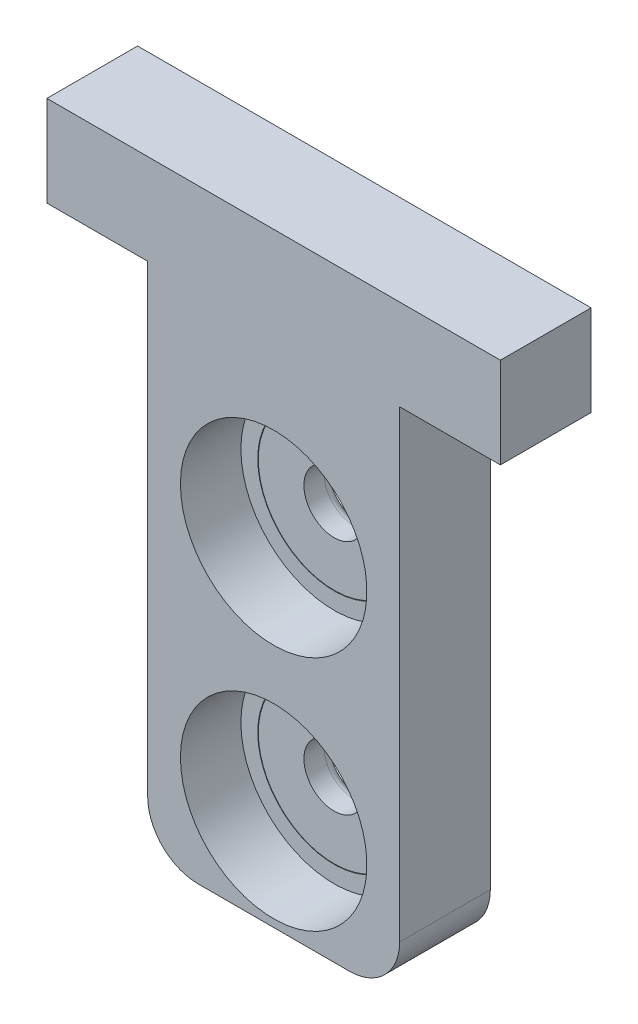
SolidWorks part; units mm, degrees
ref_plane "前视基准面" through (0, 0, 0) normal (0, 0, 1) x (1, 0, 0)
ref_plane "上视基准面" through (0, 0, 0) normal (0, 1, 0) x (1, 0, 0)
ref_plane "右视基准面" through (0, 0, 0) normal (1, 0, 0) x (0, 0, -1)
sketch "草图1" plane through (0, 0, 0) normal (0, 0, 1) x (1, 0, 0)
  line L1 (25, 60) -> (-25, 60)
  line L2 (25, 60) -> (25, -60)
  line L3 (25, -60) -> (-25, -60)
  line L4 (-25, 60) -> (-25, -60)
  line L5 (25, 60) -> (-25, -60) construction
  line L6 (25, -60) -> (-25, 60) construction
  point P0 (0, 0)
  dimension "D1" = 120
  dimension "D2" = 50
extrude "凸台-拉伸1" add sketch "草图1" along normal blind 18
sketch "草图2" plane through (0, 60, 0) normal (0, 1, 0) x (1, 0, 0)
  line L0 (25, 0) -> (-25, 0) construction
  line L1 (45, -18) -> (-45, -18)
  line L2 (45, -18) -> (45, 0)
  line L3 (45, 0) -> (-45, 0)
  line L4 (-45, -18) -> (-45, 0)
  line L5 (45, -18) -> (-45, 0) construction
  line L6 (45, 0) -> (-45, -18) construction
  line L7 (25, -18) -> (-25, -18) construction
  line L8 (0, -9) -> (0, 0) construction
  line L9 (-25, -18) -> (-25, 0) construction
  point P0 (0, -9)
  dimension "D1" = 20
extrude "凸台-拉伸2" add sketch "草图2" against normal blind 18
fillet "圆角1" radius 10 2 edges at (25, -60, 9) (-25, -60, 9)
sketch "草图3" plane through (0, 0, 0) normal (0, 0, -1) x (-1, 0, 0)
  line L0 (15, -60) -> (-15, -60) construction
  line L1 (0, 0) -> (0, -40) construction
  circle A0 centre (0, -40) radius 6
  dimension "D1" = 12
  dimension "D2" = 20
extrude "切除-拉伸1" cut sketch "草图3" against normal through all
sketch "草图4" plane through (0, 0, 0) normal (0, 0, -1) x (-1, 0, 0)
  circle A0 centre (0, -40) radius 15.0502
  circle A1 centre (0, -40) radius 15.1502
  dimension "D1" = 0.1
extrude "切除-拉伸2" cut sketch "草图4" against normal through all
pattern_linear "阵列(线性)1" count 2 spacing 47 along (0, 1, 0) of "切除-拉伸1", "切除-拉伸2"
fillet "圆角2" radius 2 4 edges at (-15.0502, -40, 18) (-15.0502, -40, 0) (-6, -40, 18) (-6, -40, 0)
fillet "圆角3" radius 2 4 edges at (-15.0502, 7, 0) (-6, 7, 0) (-15.0502, 7, 18) (-6, 7, 18)
sketch "草图5" plane through (0, 0, 18) normal (0, 0, -1) x (-1, 0, 0)
  circle A0 centre (0, -40) radius 18.5
  circle A1 centre (0, 7) radius 18.5
  dimension "D1" = 37
  dimension "D2" = 37
extrude "切除-拉伸3" cut sketch "草图5" along normal blind 12
